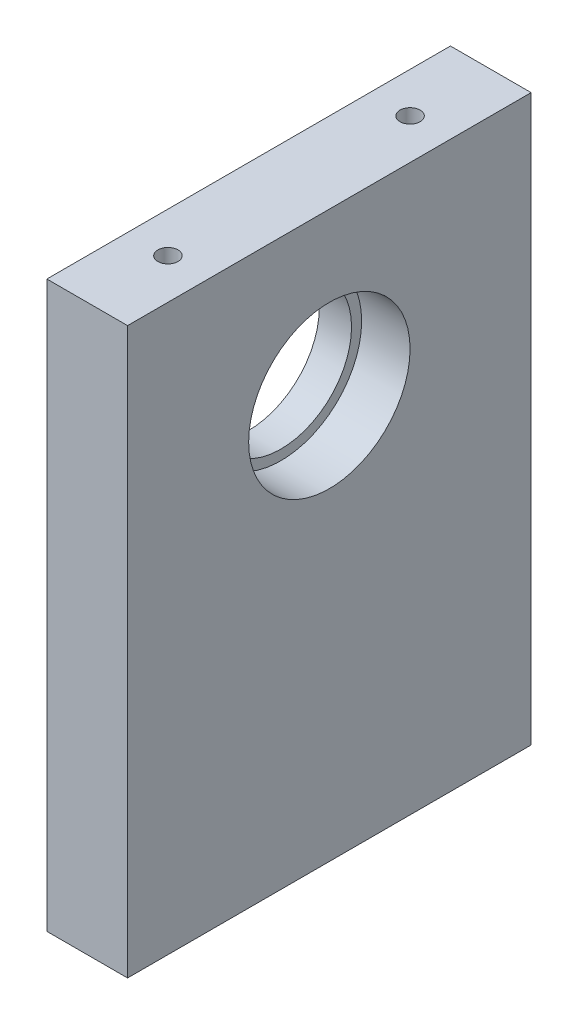
SolidWorks part; units mm, degrees
ref_plane "前视基准面" through (0, 0, 0) normal (0, 0, 1) x (1, 0, 0)
ref_plane "上视基准面" through (0, 0, 0) normal (0, 1, 0) x (1, 0, 0)
ref_plane "右视基准面" through (0, 0, 0) normal (1, 0, 0) x (0, 0, -1)
sketch "草图1" plane through (0, 0, 0) normal (1, 0, 0) x (0, 0, -1)
  line L1 (-50, 70) -> (50, 70)
  line L2 (-50, 70) -> (-50, -70)
  line L3 (-50, -70) -> (50, -70)
  line L4 (50, 70) -> (50, -70)
  line L5 (-50, 70) -> (50, -70) construction
  line L6 (-50, -70) -> (50, 70) construction
  point P0 (0, 0)
  dimension "D1" = 140
  dimension "D2" = 100
extrude "凸台-拉伸1" add sketch "草图1" along normal blind 20
hole_wizard "M10 螺纹孔1" positions "草图2" profile "草图3" tap size "M10" standard "GB"
sketch "草图2" plane through (0, -70, 0) normal (0, -1, 0) x (-1, 0, 0)
  line L0 (-10, 50) -> (-10, -79.2739)
  line L1 (-20, 50) -> (0, 50) construction
  line L3 (0, 0) -> (-46.1818, 0) construction
  point P0 (-10, 30)
  point P2 (-10, -30)
  dimension "D1" = 60
sketch "草图3" plane through (10, -70, -30) normal (1, 0, 0) x (0, 0, -1)
  line L0 (0, 0) -> (0, 27.0537)
  line L1 (0, 27.0537) -> (4.25, 24.5)
  line L2 (4.25, 24.5) -> (4.25, 0)
  line L5 (4.25, 0) -> (0, 0)
  line L10 (0, 27.0537) -> (-4.25, 24.5) construction
  line L11 (0, -6.35) -> (0, 107.95) construction
  dimension "螺纹孔钻头直径" = 8.5
  dimension "螺纹孔钻头深度" = 24.5
  dimension "导头角度" = 118
cosmetic thread "孔螺蚊线1" parameters "D1"=20, "D2"=10
cosmetic thread "孔螺蚊线2" parameters "D1"=20, "D2"=10
sketch "草图4" plane through (20, 0, 0) normal (1, 0, 0) x (0, 0, -1)
  line L0 (-50, -70) -> (50, -70) construction
  circle A0 centre (0, 30) radius 20
  dimension "D2" = 40
  dimension "D1" = 100
extrude "切除-拉伸1" cut sketch "草图4" against normal blind 12
sketch "草图5" plane through (8, 0, 0) normal (1, 0, 0) x (0, 0, -1)
  circle A0 centre (0, 30) radius 17.5
  dimension "D1" = 35
extrude "切除-拉伸2" cut sketch "草图5" against normal through all
hole_wizard "M6 螺纹孔1" positions "草图6" profile "草图7" tap size "M6" standard "GB"
sketch "草图6" plane through (0, 70, 0) normal (0, 1, 0) x (1, 0, 0)
  line L0 (0, 0) -> (41.0948, 0) construction
  line L2 (10, -50) -> (10, 58.4062) construction
  line L3 (20, -50) -> (0, -50) construction
  point P0 (10, 30)
  point P2 (10, -30)
  dimension "D1" = 60
sketch "草图7" plane through (10, 70, -30) normal (1, 0, 0) x (0, 0, 1)
  line L0 (0, 0) -> (0, 16.5022)
  line L1 (0, 16.5022) -> (2.5, 15)
  line L2 (2.5, 15) -> (2.5, 0)
  line L5 (2.5, 0) -> (0, 0)
  line L10 (0, 16.5022) -> (-2.5, 15) construction
  line L11 (0, -6.35) -> (0, 107.95) construction
  dimension "螺纹孔钻头直径" = 5
  dimension "螺纹孔钻头深度" = 15
  dimension "导头角度" = 118
cosmetic thread "孔螺蚊线3" parameters "D1"=12, "D2"=6
cosmetic thread "孔螺蚊线4" parameters "D1"=12, "D2"=6
